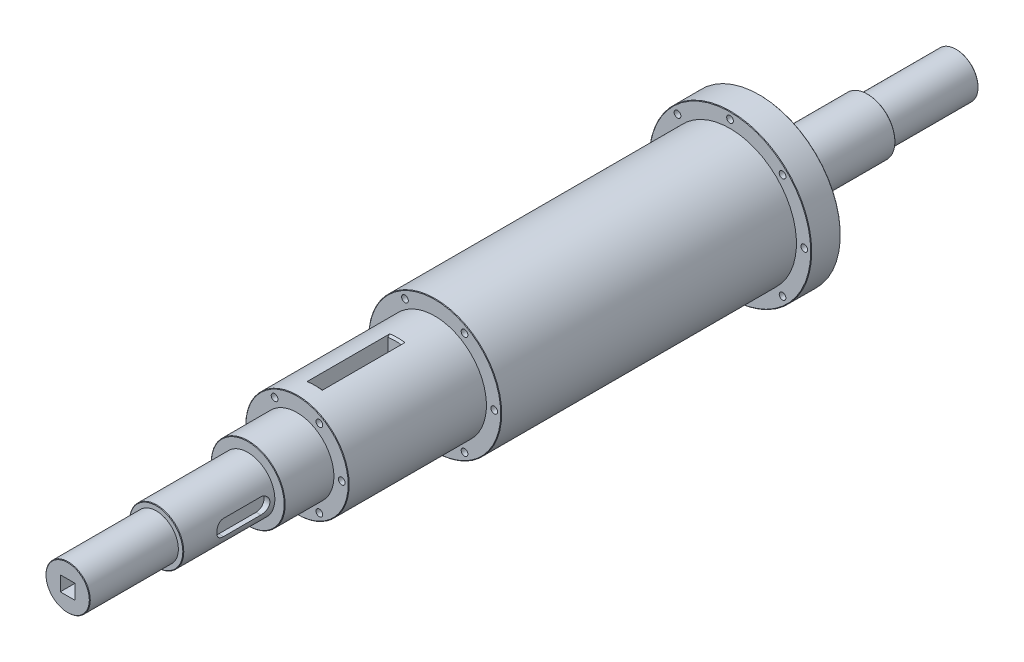
from build123d import *

# Parameters (mm, degrees)
SKETCH_3_W               = 15
SKETCH_3_H               = 15
CUT_EXTRUDE_1_DEPTH      = 911.506177903
CUT_EXTRUDE_2_DEPTH      = 576.102231468
CUT_EXTRUDE_2_DEPTH_BACK = 576.102231468
SKETCH_4_W               = 15.4
SKETCH_4_H               = 80
CHAMFER_1_SIZE           = 2
PATTERN_CIRCULAR_1_COUNT = 6
PATTERN_CIRCULAR_2_COUNT = 6
PATTERN_CIRCULAR_3_COUNT = 8
CHAMFER_2_SIZE           = 0.5
CHAMFER_3_SIZE           = 3
CHAMFER_3_SIZE2          = 5.196152423
CHAMFER_4_SIZE           = 3
CHAMFER_4_SIZE2          = 5.196152423
CUT_EXTRUDE_3_DEPTH      = 6


with BuildPart() as part:
    # 草图2 → 旋转1 (revolve)
    with BuildSketch(Plane(origin=(0, 0, 0), x_dir=(1, 0, 0), z_dir=(0, 1, 0))):
        Polygon((0, 563.143033908), (-22.5, 563.143033908), (-22.5, 473.143033908), (-28, 473.143033908), (-28, 363.143033908), (-82.5, 363.143033908), (-82.5, 333.143033908), (-67.5, 333.143033908), (-67.5, 33.143033908), (-52.5, 33.143033908), (-52.5, -106.856966092), (-37.5, -106.856966092), (-37.5, -156.856966092), (-27.5, -156.856966092), (-27.5, -249.856966092), (-22.5, -249.856966092), (-22.5, -339.856966092), (0, -339.856966092), align=None)
    revolve(axis=Axis((0, 0, 0), (0, 0, 1)))

    # 草图3 → 切除-拉伸1 (cut, through all)
    with BuildSketch(Plane(origin=(0, 0, -563.143033908), x_dir=(-1, 0, 0), z_dir=(0, 0, -1))):
        Rectangle(SKETCH_3_W, SKETCH_3_H)
    extrude(amount=-CUT_EXTRUDE_1_DEPTH, mode=Mode.SUBTRACT)

    # 草图4 → 切除-拉伸2 (cut, two sides: drawn at the far end of the back side and taken through both)
    with BuildSketch(Plane(origin=(0, 0, 0), x_dir=(1, 0, 0), z_dir=(0, 1, 0)).offset(-CUT_EXTRUDE_2_DEPTH_BACK)):
        with Locations((0, -46.856966092)):
            Rectangle(SKETCH_4_W, SKETCH_4_H)
    extrude(amount=CUT_EXTRUDE_2_DEPTH + CUT_EXTRUDE_2_DEPTH_BACK, mode=Mode.SUBTRACT)

    # 倒角1
    chamfer_1_edges = [part.edges().sort_by_distance(p)[0] for p in [
        (0, -52.5, 86.856966092),
        (0, 52.5, 86.856966092),
        (0, -52.5, 6.856966092),
        (0, 52.5, 6.856966092),
    ]]
    chamfer(chamfer_1_edges, length=CHAMFER_1_SIZE)

    # 草图6 → M8 螺纹孔1 (revolve, cut)
    with BuildSketch(Plane(origin=(-45.5, 0, 106.856966092), x_dir=(0, -1, 0), z_dir=(1, 0, 0))):
        Polygon((0, 0), (0, 21.792926105), (3.4, 19.75), (3.4, 0), align=None)
    hole_wizard_m8_1 = revolve(axis=Axis((-45.5, 0, 113.206966092), (0, 0, -1)), mode=Mode.SUBTRACT)

    # 阵列(圆周)1: M8 螺纹孔1 ×6 about axis
    pattern_circular_1_axis = Axis((0, 0, 0), (0, 0, 1))
    for i in range(1, PATTERN_CIRCULAR_1_COUNT):
        add(hole_wizard_m8_1.rotate(pattern_circular_1_axis, i * 360 / PATTERN_CIRCULAR_1_COUNT), mode=Mode.SUBTRACT)

    # 草图9 → M8 螺纹孔2 (revolve, cut)
    with BuildSketch(Plane(origin=(60.5, 0, -33.143033908), x_dir=(0, -1, 0), z_dir=(1, 0, 0))):
        Polygon((0, 0), (0, 21.792926105), (3.4, 19.75), (3.4, 0), align=None)
    hole_wizard_m8_2 = revolve(axis=Axis((60.5, 0, -26.793033908), (0, 0, -1)), mode=Mode.SUBTRACT)

    # 阵列(圆周)2: M8 螺纹孔2 ×6 about axis
    pattern_circular_2_axis = Axis((0, 0, 0), (0, 0, 1))
    for i in range(1, PATTERN_CIRCULAR_2_COUNT):
        add(hole_wizard_m8_2.rotate(pattern_circular_2_axis, i * 360 / PATTERN_CIRCULAR_2_COUNT), mode=Mode.SUBTRACT)

    # 草图11 → M8 螺纹孔3 (revolve, cut)
    with BuildSketch(Plane(origin=(-75.5, 0, -333.143033908), x_dir=(0, -1, 0), z_dir=(1, 0, 0))):
        Polygon((0, 0), (0, 21.792926105), (3.4, 19.75), (3.4, 0), align=None)
    hole_wizard_m8_3 = revolve(axis=Axis((-75.5, 0, -326.793033908), (0, 0, -1)), mode=Mode.SUBTRACT)

    # 阵列(圆周)3: M8 螺纹孔3 ×8 about axis
    pattern_circular_3_axis = Axis((0, 0, 0), (0, 0, 1))
    for i in range(1, PATTERN_CIRCULAR_3_COUNT):
        add(hole_wizard_m8_3.rotate(pattern_circular_3_axis, i * 360 / PATTERN_CIRCULAR_3_COUNT), mode=Mode.SUBTRACT)

    # 倒角2
    chamfer_2_edges = [part.edges().sort_by_distance(p)[0] for p in [
        (22.5, 0, 339.856966092),
        (27.5, 0, 249.856966092),
        (37.5, 0, 156.856966092),
        (52.5, 0, 106.856966092),
        (67.5, 0, -33.143033908),
        (82.5, 0, -333.143033908),
        (82.5, 0, -363.143033908),
        (28, 0, -473.143033908),
        (22.5, 0, -563.143033908),
    ]]
    chamfer(chamfer_2_edges, length=CHAMFER_2_SIZE)

    # 倒角3
    chamfer_3_edges = [part.edges().sort_by_distance(p)[0] for p in [
        (-7.5, 0, -563.143033908),
        (0, 7.5, -563.143033908),
        (7.5, 0, -563.143033908),
        (0, -7.5, -563.143033908),
    ]]
    chamfer_3_side = [part.faces().sort_by_distance(p)[0] for p in [
        (21.377746033, 0, -563.143033908),
    ]]
    chamfer(chamfer_3_edges, length=CHAMFER_3_SIZE, length2=CHAMFER_3_SIZE2, reference=chamfer_3_side[0])

    # 倒角4
    chamfer_4_edges = [part.edges().sort_by_distance(p)[0] for p in [
        (0, 7.5, 86.856966092),
        (0, -7.5, 86.856966092),
    ]]
    chamfer_4_side = [part.faces().sort_by_distance(p)[0] for p in [
        (-7.597832686, 0, 86.856966092),
    ]]
    chamfer(chamfer_4_edges, length=CHAMFER_4_SIZE, length2=CHAMFER_4_SIZE2, reference=chamfer_4_side[0])

    # 草图12 → 切除-拉伸3 (cut)
    with BuildSketch(Plane(origin=(27.5, 0, 0), x_dir=(0, 0, -1), z_dir=(1, 0, 0))):
        with BuildLine():
            Line((-169.856966092, -8), (-207.856966092, -8))
            ThreePointArc((-207.856966092, -8), (-215.856966092, 0), (-207.856966092, 8))
            Line((-207.856966092, 8), (-169.856966092, 8))
            ThreePointArc((-169.856966092, 8), (-161.856966092, 0), (-169.856966092, -8))
        make_face()
    extrude(amount=-CUT_EXTRUDE_3_DEPTH, mode=Mode.SUBTRACT)


solid = part.part
